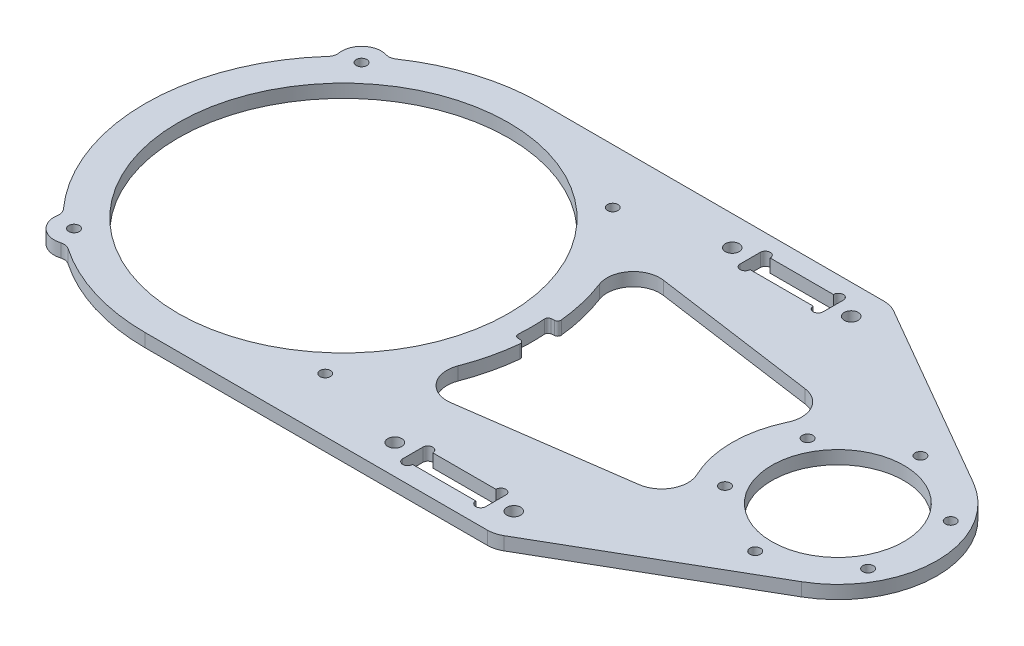
from build123d import *

# Parameters (mm, degrees)
SKETCH_1_R      = 50
SKETCH_1_R_2    = 20
SKETCH_1_R_3    = 1.6
SKETCH_1_R_4    = 2.1
EXTRUDE_1_DEPTH = 4
FILLET_R8_1_R   = 8
FILLET_R2_2_R   = 1
FILLET_R3_R     = 3


with BuildPart() as part:
    # 草图1 → 凸台-拉伸1 (new body)
    with BuildSketch(Plane(origin=(0, 0, 0), x_dir=(1, 0, 0), z_dir=(0, 1, 0))):
        with BuildLine():
            Line((21.076951546, 60), (80, 25.980762114))
            ThreePointArc((80, 25.980762114), (95, 0), (80, -25.980762114))
            Line((80, -25.980762114), (21.076951546, -60))
            Line((21.076951546, -60), (-84.599054368, -60))
            ThreePointArc((-84.599054368, -60), (-103.000462095, -57.108564977), (-119.628320662, -48.712939789))
            ThreePointArc((-119.628320662, -48.712939789), (-126.546403622, -48.018676119), (-128.163868254, -41.256599364))
            ThreePointArc((-128.163868254, -41.256599364), (-144.599054368, 0), (-128.163868254, 41.256599364))
            ThreePointArc((-128.163868254, 41.256599364), (-126.546403622, 48.018676119), (-119.628320662, 48.712939789))
            ThreePointArc((-119.628320662, 48.712939789), (-103.000462095, 57.108564977), (-84.599054368, 60))
            Line((-84.599054368, 60), (21.076951546, 60))
        make_face()
        with Locations(Location((-84.599054368, 0, 0), (0, 0, 270))):
            Circle(SKETCH_1_R, mode=Mode.SUBTRACT)
        with Locations(Location((65, 0, 0), (0, 0, 270))):
            Circle(SKETCH_1_R_2, mode=Mode.SUBTRACT)
        with Locations(Location((65, 25, 0), (0, 0, 270))):
            Circle(SKETCH_1_R_3, mode=Mode.SUBTRACT)
        with Locations(Location((86.650635095, 12.5, 0), (0, 0, 270))):
            Circle(SKETCH_1_R_3, mode=Mode.SUBTRACT)
        with Locations(Location((86.650635095, -12.5, 0), (0, 0, 270))):
            Circle(SKETCH_1_R_3, mode=Mode.SUBTRACT)
        with Locations(Location((65, -25, 0), (0, 0, 270))):
            Circle(SKETCH_1_R_3, mode=Mode.SUBTRACT)
        with Locations(Location((43.349364905, -12.5, 0), (0, 0, 270))):
            Circle(SKETCH_1_R_3, mode=Mode.SUBTRACT)
        with Locations(Location((43.349364905, 12.5, 0), (0, 0, 270))):
            Circle(SKETCH_1_R_3, mode=Mode.SUBTRACT)
        with Locations(Location((-18, 51.05, 0), (0, 0, 270))):
            Circle(SKETCH_1_R_4, mode=Mode.SUBTRACT)
        with Locations(Location((18, 51.05, 0), (0, 0, 270))):
            Circle(SKETCH_1_R_4, mode=Mode.SUBTRACT)
        with Locations(Location((-18, -51.05, 0), (0, 0, 90))):
            Circle(SKETCH_1_R_4, mode=Mode.SUBTRACT)
        with Locations(Location((18, -51.05, 0), (0, 0, 90))):
            Circle(SKETCH_1_R_4, mode=Mode.SUBTRACT)
        with Locations(Location((-46.599054368, 43.5, 0), (0, 0, 270))):
            Circle(SKETCH_1_R_3, mode=Mode.SUBTRACT)
        with Locations(Location((-122.599054368, 43.5, 0), (0, 0, 90))):
            Circle(SKETCH_1_R_3, mode=Mode.SUBTRACT)
        with Locations(Location((-46.599054368, -43.5, 0), (0, 0, 90))):
            Circle(SKETCH_1_R_3, mode=Mode.SUBTRACT)
        with Locations(Location((-122.599054368, -43.5, 0), (0, 0, 270))):
            Circle(SKETCH_1_R_3, mode=Mode.SUBTRACT)
        with BuildLine():
            Line((-9.55, 54.1), (9.55, 54.1))
            ThreePointArc((9.55, 54.1), (11.05, 55.6), (12.55, 54.1))
            Line((12.55, 54.1), (12.55, 48))
            ThreePointArc((12.55, 48), (11.05, 46.5), (9.55, 48))
            Line((9.55, 48), (-9.55, 48))
            ThreePointArc((-9.55, 48), (-11.05, 46.5), (-12.55, 48))
            Line((-12.55, 48), (-12.55, 54.1))
            ThreePointArc((-12.55, 54.1), (-11.05, 55.6), (-9.55, 54.1))
        make_face(mode=Mode.SUBTRACT)
        with BuildLine():
            Line((-9.55, -48), (9.55, -48))
            ThreePointArc((9.55, -48), (11.05, -46.5), (12.55, -48))
            Line((12.55, -48), (12.55, -54.1))
            ThreePointArc((12.55, -54.1), (11.05, -55.6), (9.55, -54.1))
            Line((9.55, -54.1), (-9.55, -54.1))
            ThreePointArc((-9.55, -54.1), (-11.05, -55.6), (-12.55, -54.1))
            Line((-12.55, -54.1), (-12.55, -48))
            ThreePointArc((-12.55, -48), (-11.05, -46.5), (-9.55, -48))
        make_face(mode=Mode.SUBTRACT)
        with BuildLine():
            Line((-35.371920456, 34.302904932), (43.046573591, 23.281904323))
            ThreePointArc((43.046573591, 23.281904323), (33, 0), (43.046573591, -23.281904323))
            Line((43.046573591, -23.281904323), (-35.371920456, -34.302904932))
            ThreePointArc((-35.371920456, -34.302904932), (-28.194236848, -20.457188481), (-24.827372483, -5.229344565))
            Line((-24.827372483, -5.229344565), (-27.815956577, -4.967877337))
            ThreePointArc((-27.815956577, -4.967877337), (-27.599054368, 0), (-27.815956577, 4.967877337))
            Line((-27.815956577, 4.967877337), (-24.827372483, 5.229344565))
            ThreePointArc((-24.827372483, 5.229344565), (-28.194236848, 20.457188481), (-35.371920456, 34.302904932))
        make_face(mode=Mode.SUBTRACT)
    extrude(amount=EXTRUDE_1_DEPTH)

    # R8 圆角1
    fillet_r8_1_edges = [part.edges().sort_by_distance(p)[0] for p in [
        (-35.371920456, 2, -34.302904932),
        (-35.371920456, 2, 34.302904932),
        (43.046573591, 2, 23.281904323),
        (43.046573591, 2, -23.281904323),
        (21.076951546, 2, -60),
        (21.076951546, 2, 60),
    ]]
    fillet(fillet_r8_1_edges, radius=FILLET_R8_1_R)

    # R2 圆角2
    fillet_r2_2_edges = [part.edges().sort_by_distance(p)[0] for p in [
        (-24.827372483, 2, -5.229344565),
        (-27.815956577, 2, -4.967877337),
        (-27.815956577, 2, 4.967877337),
        (-24.827372483, 2, 5.229344565),
    ]]
    fillet(fillet_r2_2_edges, radius=FILLET_R2_2_R)

    # R3 圆角
    fillet_r3_edges = [part.edges().sort_by_distance(p)[0] for p in [
        (-119.628320662, 2, 48.712939789),
        (-128.163868254, 2, 41.256599364),
        (-128.163868254, 2, -41.256599364),
        (-119.628320662, 2, -48.712939789),
    ]]
    fillet(fillet_r3_edges, radius=FILLET_R3_R)


solid = part.part
